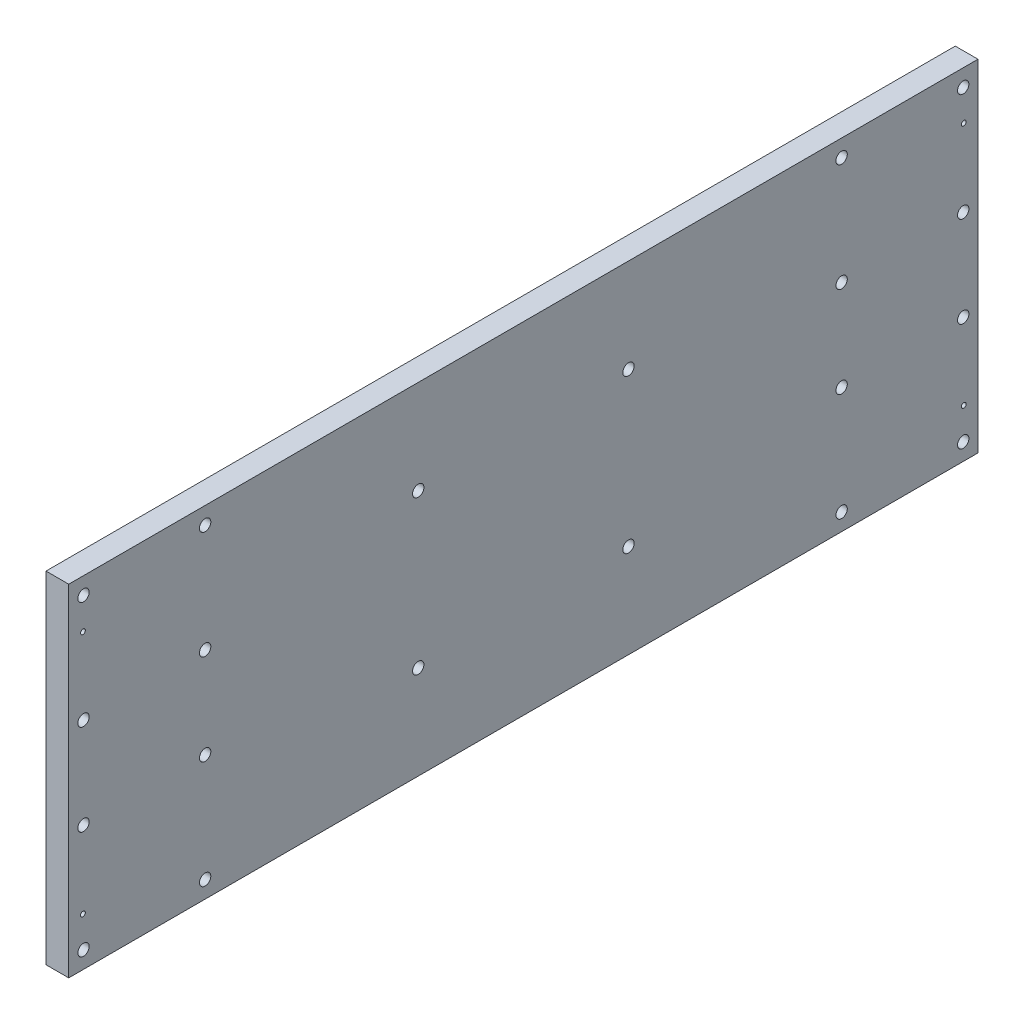
from build123d import *

# Parameters (mm, degrees)
SKETCH1_W           = 800
SKETCH1_H           = 300
BOSS_EXTRUDE1_DEPTH = 20
SKETCH2_R           = 5
CUT_EXTRUDE1_DEPTH  = 20
SKETCH3_R           = 2.1
CUT_EXTRUDE2_DEPTH  = 65
SKETCH4_R           = 5
CUT_EXTRUDE3_DEPTH  = 226


with BuildPart() as part:
    # Sketch1 → Boss-Extrude1 (new body)
    with BuildSketch(Plane(origin=(0, 0, 0), x_dir=(0, 0, -1), z_dir=(1, 0, 0))):
        Rectangle(SKETCH1_W, SKETCH1_H)
    extrude(amount=BOSS_EXTRUDE1_DEPTH)

    # Sketch2 → Cut-Extrude1 (cut)
    with BuildSketch(Plane(origin=(20, 0, 0), x_dir=(0, 0, -1), z_dir=(1, 0, 0))):
        with Locations((-387, 135)):
            Circle(SKETCH2_R)
        with Locations((-280, 135)):
            Circle(SKETCH2_R)
        with Locations((-280, 40)):
            Circle(SKETCH2_R)
        with Locations((-387, 40)):
            Circle(SKETCH2_R)
        with Locations(Location((-280, -40, 0), (0, 0, 180))):
            Circle(SKETCH2_R)
        with Locations(Location((-280, -135, 0), (0, 0, 180))):
            Circle(SKETCH2_R)
        with Locations(Location((-387, -135, 0), (0, 0, 180))):
            Circle(SKETCH2_R)
        with Locations(Location((-387, -40, 0), (0, 0, 180))):
            Circle(SKETCH2_R)
        with Locations((280, -40)):
            Circle(SKETCH2_R)
        with Locations((280, -135)):
            Circle(SKETCH2_R)
        with Locations((387, -135)):
            Circle(SKETCH2_R)
        with Locations((387, -40)):
            Circle(SKETCH2_R)
        with Locations(Location((280, 135, 0), (0, 0, 180))):
            Circle(SKETCH2_R)
        with Locations(Location((387, 135, 0), (0, 0, 180))):
            Circle(SKETCH2_R)
        with Locations(Location((387, 40, 0), (0, 0, 180))):
            Circle(SKETCH2_R)
        with Locations(Location((280, 40, 0), (0, 0, 180))):
            Circle(SKETCH2_R)
    extrude(amount=-CUT_EXTRUDE1_DEPTH, mode=Mode.SUBTRACT)

    # Sketch3 → Cut-Extrude2 (cut)
    with BuildSketch(Plane(origin=(20, 0, 0), x_dir=(0, 0, -1), z_dir=(1, 0, 0))):
        with Locations((387.5, -107.5)):
            Circle(SKETCH3_R)
        with Locations(Location((387.5, 107.5, 0), (0, 0, 180))):
            Circle(SKETCH3_R)
        with Locations(Location((-387.5, -107.5, 0), (0, 0, 180))):
            Circle(SKETCH3_R)
        with Locations((-387.5, 107.5)):
            Circle(SKETCH3_R)
    extrude(amount=-CUT_EXTRUDE2_DEPTH, mode=Mode.SUBTRACT)

    # Sketch4 → Cut-Extrude3 (cut)
    with BuildSketch(Plane(origin=(20, 0, 0), x_dir=(0, 0, -1), z_dir=(1, 0, 0))):
        with Locations((-92.5, 67.5)):
            Circle(SKETCH4_R)
        with Locations((92.5, 67.5)):
            Circle(SKETCH4_R)
        with Locations((92.5, -67.5)):
            Circle(SKETCH4_R)
        with Locations((-92.5, -67.5)):
            Circle(SKETCH4_R)
    extrude(amount=-CUT_EXTRUDE3_DEPTH, mode=Mode.SUBTRACT)


solid = part.part
